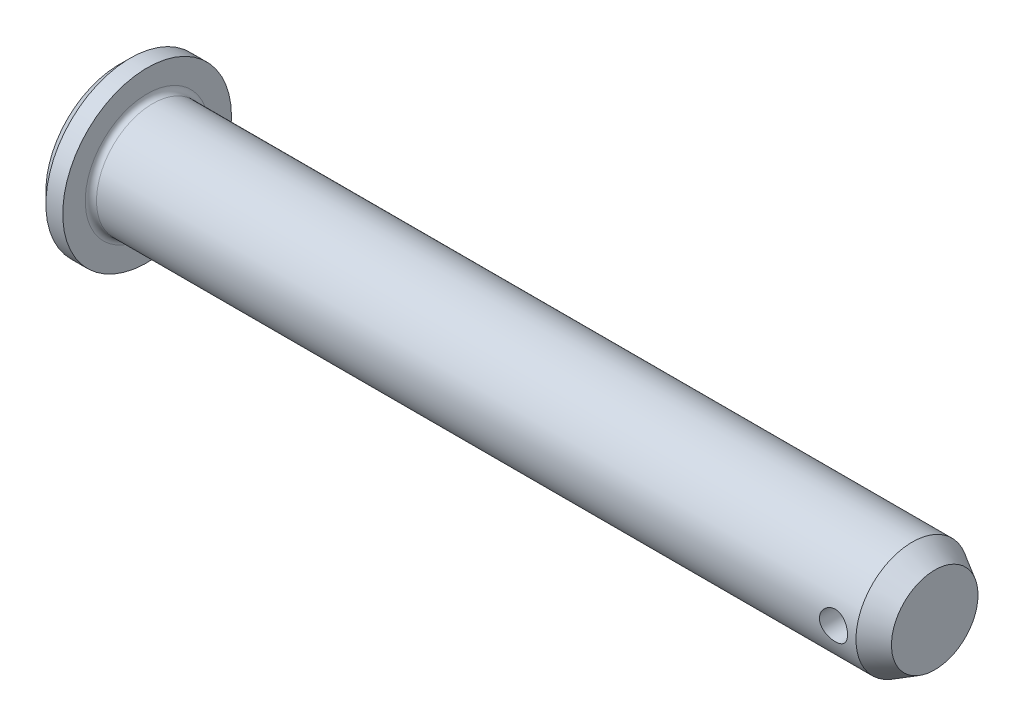
from build123d import *

# Parameters (mm, degrees)
CUT_EXTRUDE_1_DEPTH      = 147.543508898
CUT_EXTRUDE_1_DEPTH_BACK = 147.543508898
SKETCH_2_R               = 2.5
FILLET_1_R               = 1
CHAMFER_1_SIZE           = 4
CHAMFER_1_SIZE2          = 2.309401077


with BuildPart() as part:
    # 草图1 → Revolve 546 (revolve)
    with BuildSketch(Plane.XY, mode=Mode.PRIVATE) as revolve_546_sk:
        Polygon((0, 0), (145, 0), (145, 10), (5, 10), (5, 15), (2, 15), (0, 13), align=None)
    revolve(revolve_546_sk.sketch.rotate(Axis((0, 0, 0), (-1, 0, 0)), 90), axis=Axis((0, 0, 0), (-1, 0, 0)))

    # 草图2 → 切除-拉伸1 (cut, two sides: drawn at the far end of the back side and taken through both)
    with BuildSketch(Plane.XY.offset(-CUT_EXTRUDE_1_DEPTH_BACK)):
        with Locations((137, 0)):
            Circle(SKETCH_2_R)
    extrude(amount=CUT_EXTRUDE_1_DEPTH + CUT_EXTRUDE_1_DEPTH_BACK, mode=Mode.SUBTRACT)

    # 圆角1
    fillet_1_edges = [part.edges().sort_by_distance(p)[0] for p in [
        (5, 0, 10),
    ]]
    fillet(fillet_1_edges, radius=FILLET_1_R)

    # 倒角1
    chamfer_1_edges = [part.edges().sort_by_distance(p)[0] for p in [
        (145, 0, 10),
    ]]
    chamfer_1_side = [part.faces().sort_by_distance(p)[0] for p in [
        (75.5, 0, 10),
    ]]
    chamfer(chamfer_1_edges, length=CHAMFER_1_SIZE, length2=CHAMFER_1_SIZE2, reference=chamfer_1_side[0])


solid = part.part
